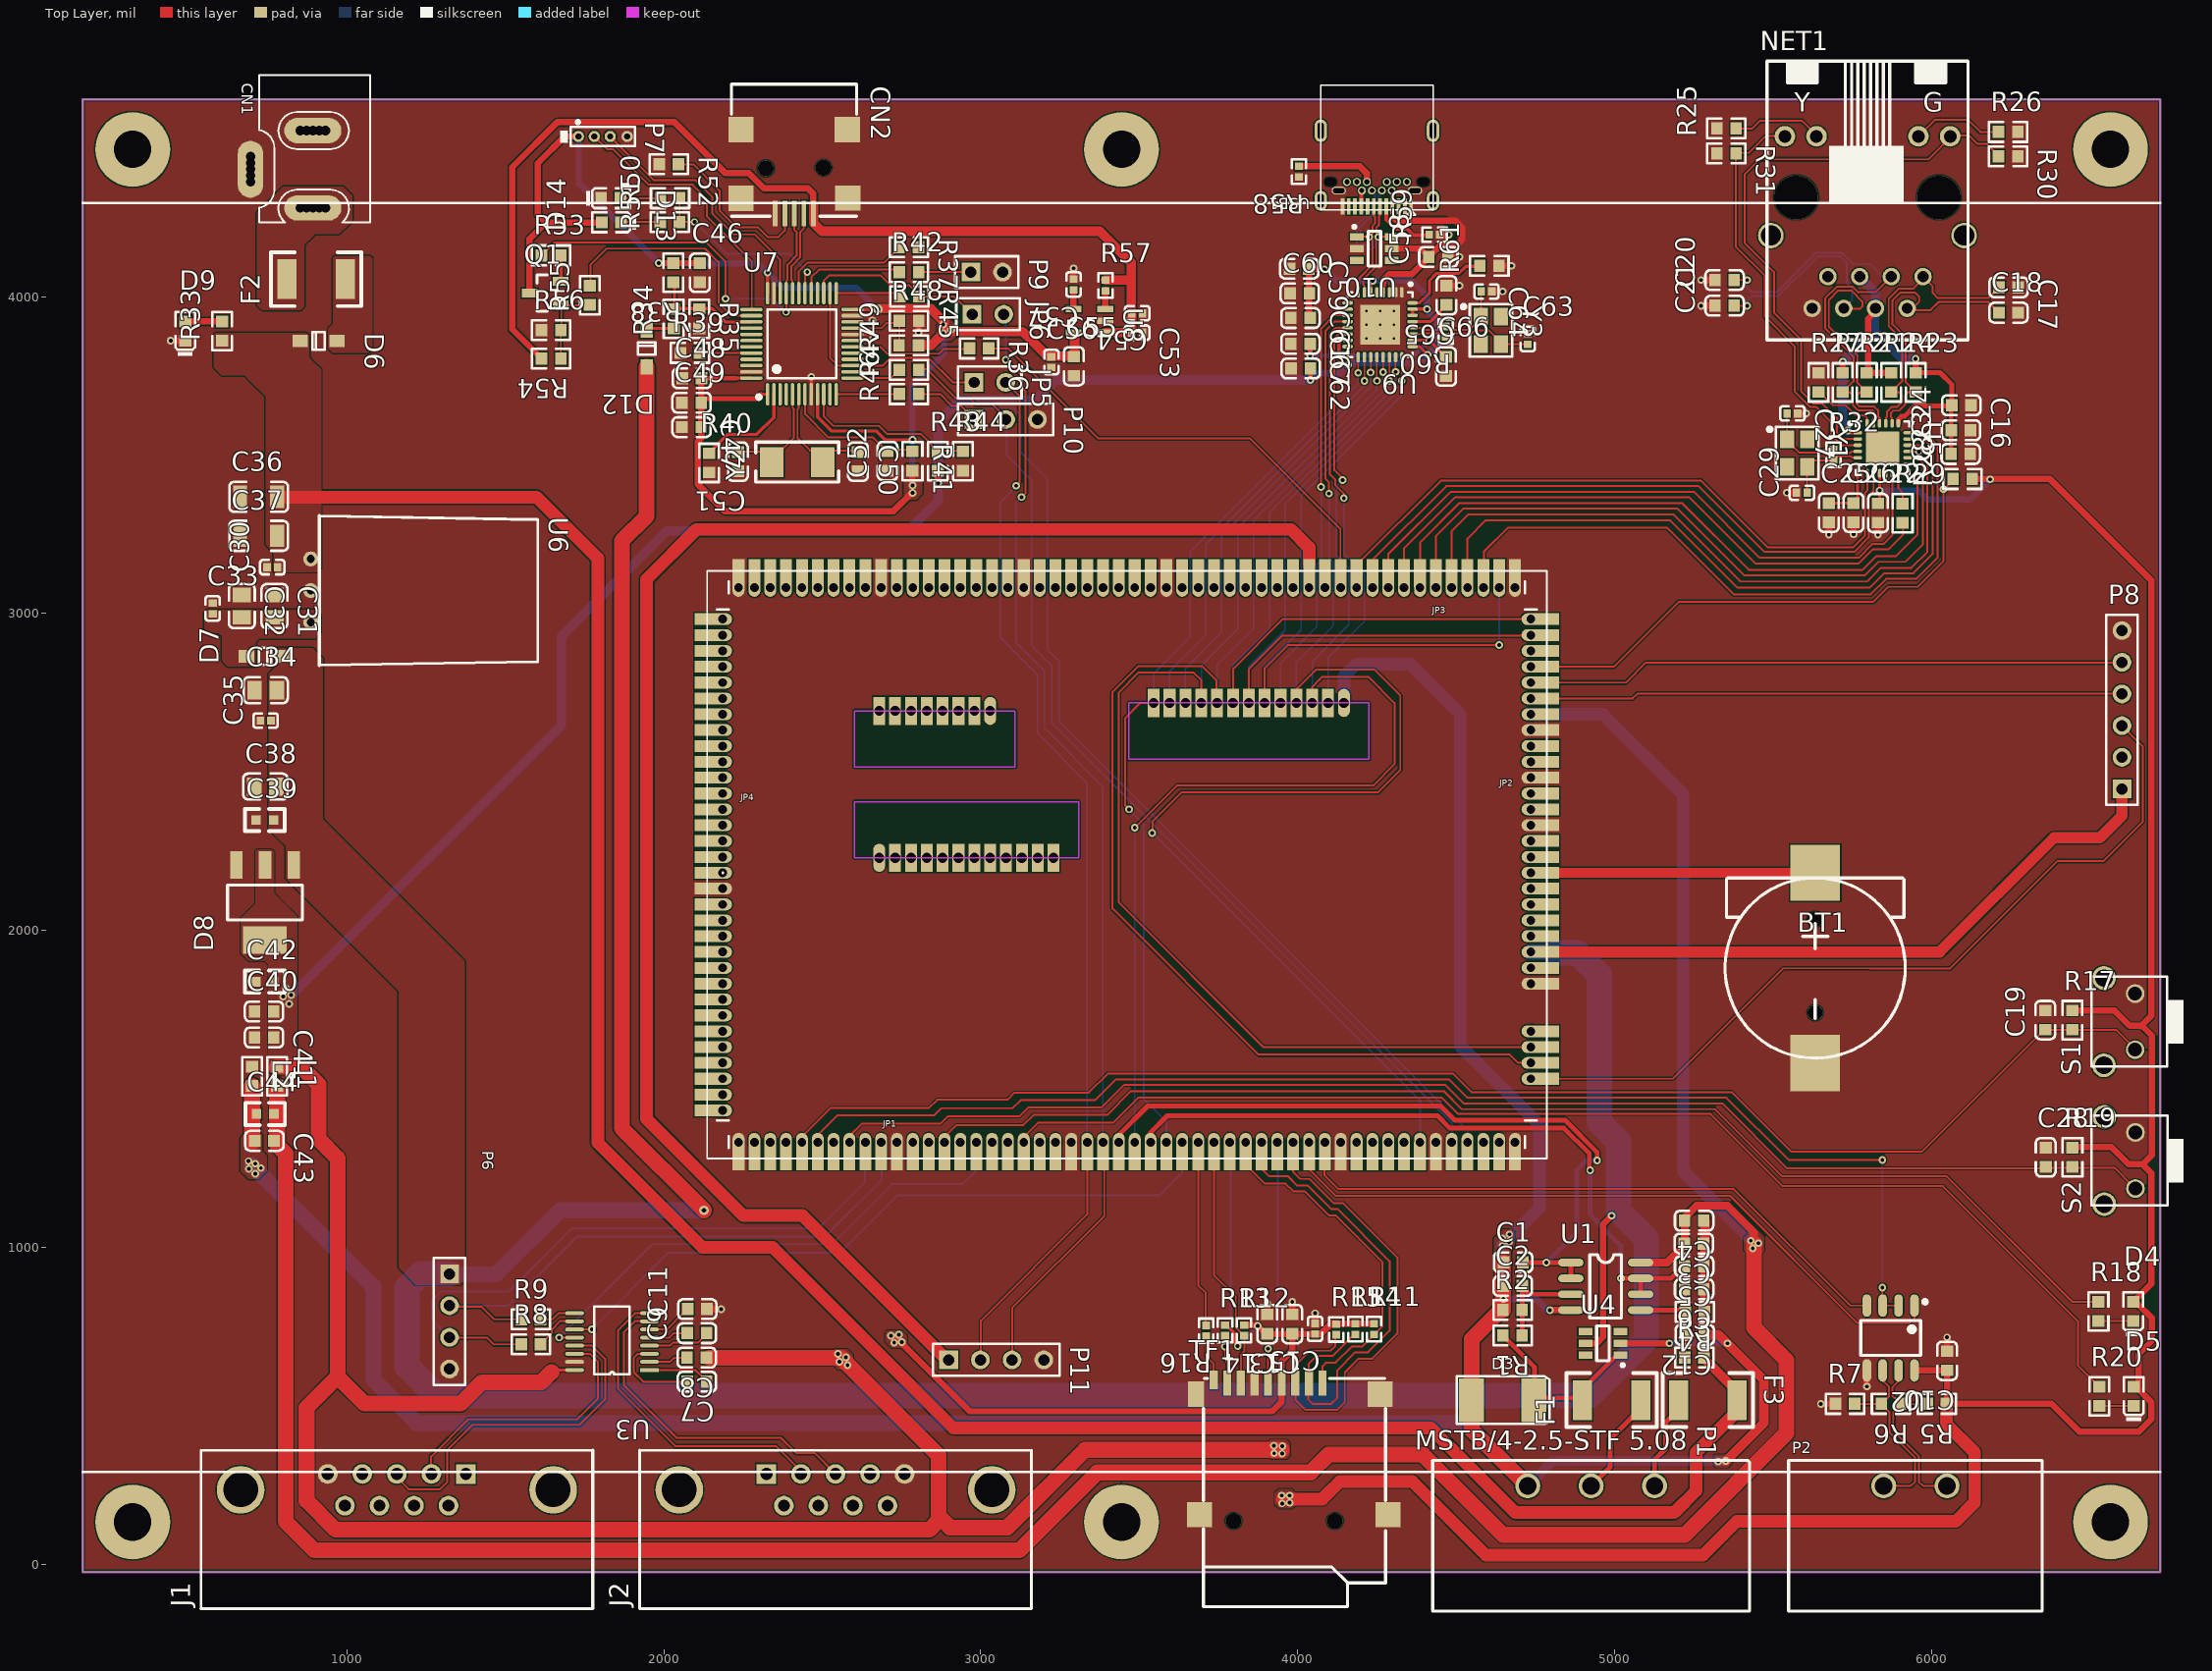
[diagram p0: Top Layer view]
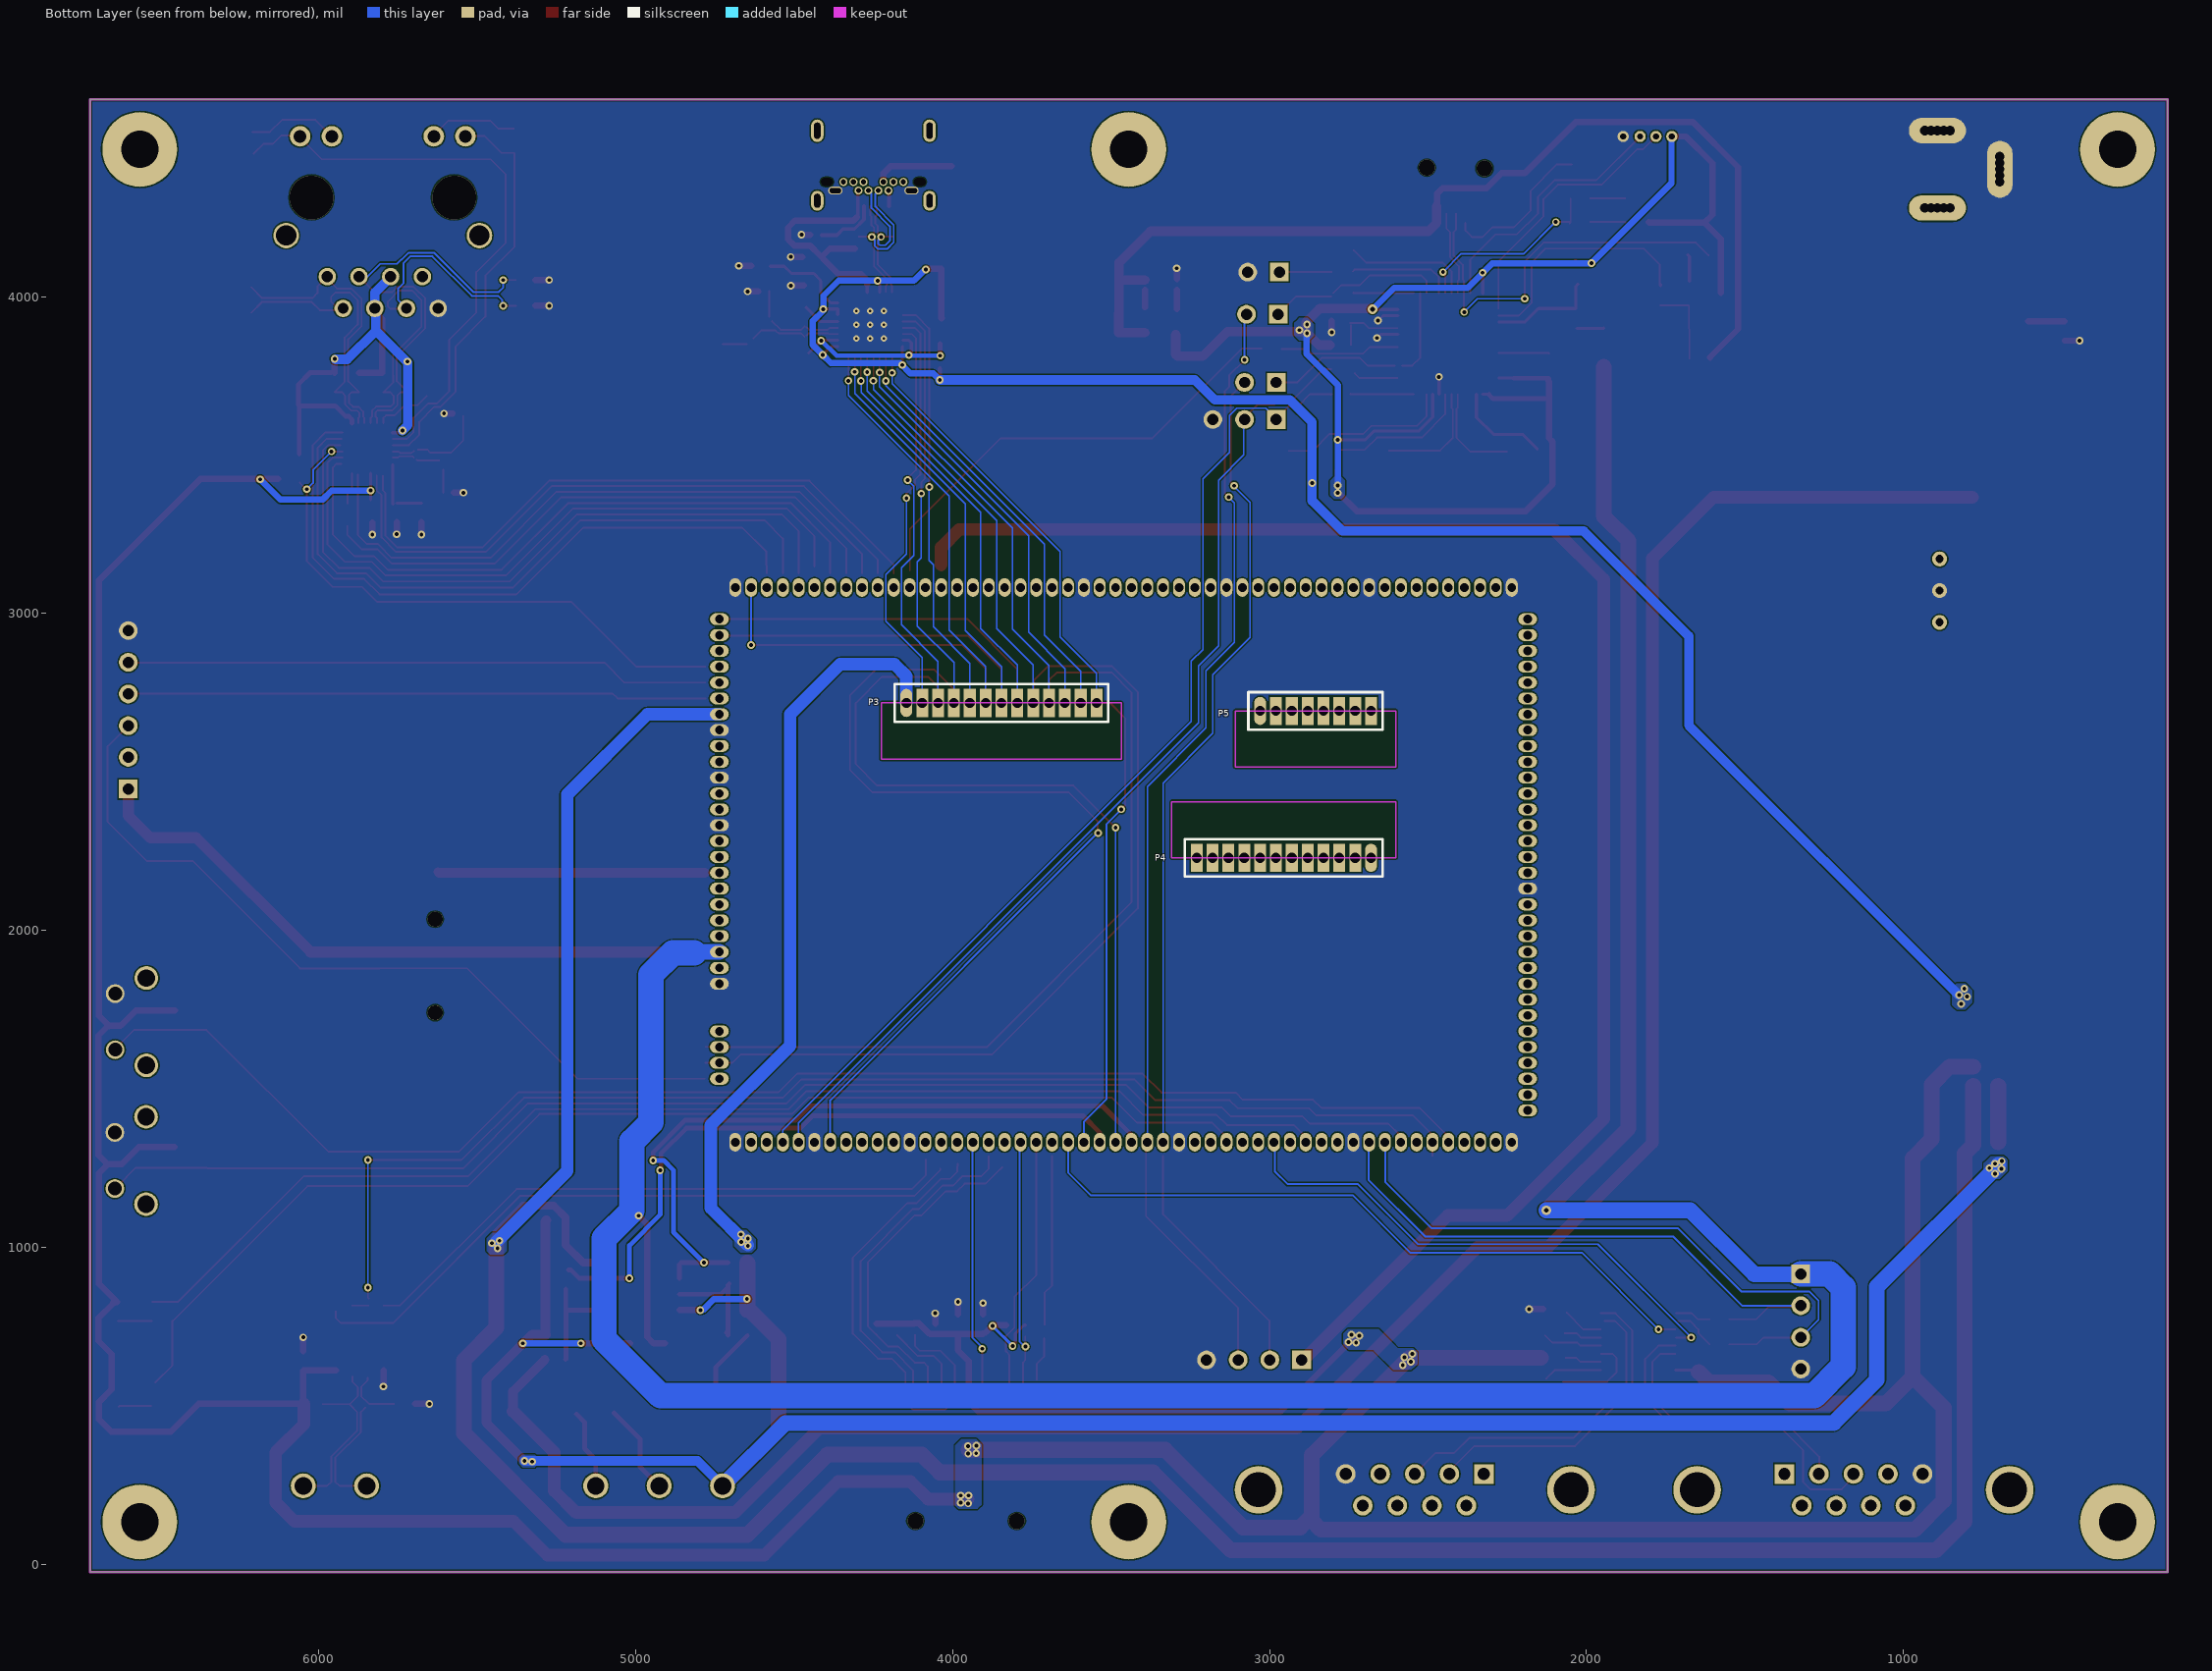
[diagram p1: Bottom Layer view, seen from below]
# Altium PCB MISC105202-15.PcbDoc (part 1 of 4)
Units mil, origin at the board's own origin, x right, y up, seen from the top; angles counter-clockwise.
Board outline 6555.12 x 4645.67 mil, 2 copper layers (Top Layer, Bottom Layer); 182 components, 258 nets, 994 pads, 145 vias.
Unrouted connection lines stored in the file: 1.

## Layer stack, top to bottom (the 12.6 mil dielectric is the usual default, probably not edited)
Top Layer: signal copper 1.4
Dielectric: dielectric 12.6, FR-4, Dk 4.8
Bottom Layer: signal copper 1.4

## Board outline
167,-24 167,4621.67 6722.12,4621.67 6722.12,-24

## Design rules (kind name [scope] priority, off if disabled: settings)
Clearance [All] p1: gap=4
ComponentClearance [All] p1: gap=10 collisioncheckmode=3 verticalgap=0 showdistances=FALSE
DiffPairsRouting [All] p1: maxlimit=6 minlimit=6 mostfreqgap=6 maxuncoupledlength=500
FanoutControl Fanout_Small [All] p1 off: bgadir=Out bgaviamode=Centered fanoutstyle=Auto fanoutdirection=Alternating viagrid=1 // Protel DXP Scope 1 Expression Was: (CompPinCount < 5)   Fanout_Small (Default Rule)
FanoutControl Fanout_Default [All] p2: bgadir=Out bgaviamode=Centered fanoutstyle=Auto fanoutdirection=Alternating viagrid=1 // Fanout_Default (Default Rule)
FanoutControl Fanout_SOIC [All] p3 off: bgadir=Out bgaviamode=Centered fanoutstyle=Auto fanoutdirection=Alternating viagrid=1 // Protel DXP Scope 1 Expression Was: IsSOIC   Fanout_SOIC (Default Rule)
FanoutControl Fanout_BGA [All] p4 off: bgadir=Out bgaviamode=Centered fanoutstyle=Auto fanoutdirection=Alternating viagrid=1 // Protel DXP Scope 1 Expression Was: IsBGA   Fanout_BGA (Default Rule)
FanoutControl Fanout_LCC [All] p5 off: bgadir=Out bgaviamode=Centered fanoutstyle=Auto fanoutdirection=Alternating viagrid=1 // Protel DXP Scope 1 Expression Was: IsLCC   Fanout_LCC (Default Rule)
MatchedLengths "Schematic Matched Net Lengths_8" [InNet('TD_N')] p1: tolerance=100 checknetsindiffpair=TRUE checkdiffpairvsdiffpair=TRUE checkothers=TRUE
MatchedLengths "Schematic Matched Net Lengths_7" [InNet('TD_N')] p2: tolerance=100 checknetsindiffpair=TRUE checkdiffpairvsdiffpair=TRUE checkothers=TRUE
MatchedLengths "Schematic Matched Net Lengths_6" [InNet('TD_N')] p3: tolerance=100 checknetsindiffpair=TRUE checkdiffpairvsdiffpair=TRUE checkothers=TRUE
MatchedLengths "Schematic Matched Net Lengths_5" [InNet('TD_P')] p4: tolerance=100 checknetsindiffpair=TRUE checkdiffpairvsdiffpair=TRUE checkothers=TRUE
MatchedLengths "Schematic Matched Net Lengths_4" [InNet('TD_P')] p5: tolerance=100 checknetsindiffpair=TRUE checkdiffpairvsdiffpair=TRUE checkothers=TRUE
MatchedLengths "Schematic Matched Net Lengths_3" [InNet('TD_N')] p6: tolerance=100 checknetsindiffpair=TRUE checkdiffpairvsdiffpair=TRUE checkothers=TRUE
MatchedLengths "Schematic Matched Net Lengths_2" [InNet('TD_N')] p7: tolerance=100 checknetsindiffpair=TRUE checkdiffpairvsdiffpair=TRUE checkothers=TRUE
MatchedLengths "Schematic Matched Net Lengths_1" [InNet('RD_P')] p8: tolerance=100 checknetsindiffpair=TRUE checkdiffpairvsdiffpair=TRUE checkothers=TRUE
MatchedLengths "Schematic Matched Net Lengths" [InNet('RD_N')] p9: tolerance=100 checknetsindiffpair=TRUE checkdiffpairvsdiffpair=TRUE checkothers=TRUE
MinimumSolderMaskSliver [All] p1: minsoldermaskwidth=0
PolygonConnect [All] p1: connectstyle=Direct reliefconductorwidth=10 reliefentries=4 polygonreliefangle="90 Angle"
RoutingVias [All] p1: holewidth=12 width=24 viastyle="Through Hole" minholewidth=12 minwidth=24 maxholewidth=12 maxwidth=24
SilkToSilkClearance [All] p1: silktosilkclearance=0
SilkscreenOverComponentPads SilkToSolderMaskClearance [IsPad] p1 off: minsilkscreentomaskgap=0 // Protel DXP Scope 1 Expression Was: IsPad
SolderMaskExpansion [All] p1: expansion=4
Width [All] p1: maxlimit=80 minlimit=4 preferedwidth=6 toplayer_minwidth=6 minimp=50.000000 maximp=50.000000 favimp=50.000000
18 further rules are at their usual default settings.

## Classes and differential pairs
component class ADC_Exp: C1 C2 C3 C4 C5 C6 C12 D3 F1 F3 P1 R1 R2 R3 R4 U1 U4
component class Connect: C7 C8 C9 C10 C11 C13 C14 C15 J1 J2 P2 P6 R5 R6 R7 R8 R9 R11 R12 R13 R14 R15 R16 TF1 U2 U3
component class Core: C19 C28 D4 D5 JP1 JP2 JP3 JP4 P3 P4 P5 P8 P11 R17 R18 R19 R20 S1 S2
component class Ethernet: C16 C17 C18 C20 C21 C22 C23 C24 C25 C26 C27 C29 NET1 R21 R22 R23 R24 R25 R26 R27 R28 R29 R30 R31 R32 U5 Y1
component class PWR: BT1 C30 C31 C32 C33 C34 C35 C36 C37 C38 C39 C40 C41 C42 C43 C44 CN1 D6 D7 D8 D9 F2 L1 L2 R33 U6
component class ST_Link: C46 C47 C48 C49 C50 C51 C52 C53 C54 C55 C56 C57 CN2 D12 D13 D14 JP5 JP6 P7 P9 P10 Q1 R34 R35 R36 R37 R38 R39 R40 R41 R42 R43 R44 R45 R46 R47 R48 R49 R50 R51 R52 R53 R54 R55 R56 R57 U7 U8 Y2
component class USB: C58 C59 C60 C61 C62 C63 C64 C65 C66 C67 R58 R59 R60 R61 U9 U10 USB1 Y3
differential pair NewDifferentialPair3: +DSI_CK_N -DSI_CK_P
differential pair NewDifferentialPair2: +D_N -D_P
differential pair NewDifferentialPair1: +RS485_A -RS485_B
differential pair RD: +RD_P -RD_N
differential pair TD: +TD_P -TD_N
differential pair NewDifferentialPair4: +STLINK_USB_DM -STLINK_USB_DP

## Components (designator, comment, footprint, x,y, rotation, side; value= is the part's Value field where it differs from the comment)
BT1 "CR2032-3V" BT1 5621,1862 r90 top
C1 "100pF,50V" 0603_C 4680,953 r0 top
C2 "100pF,50V" 0603_C 4679,878 r0 top
C3 "10uF,10V" 0603_C 5250,1012 r180 top
C4 "100nF,50V" 0603_C 5251,1084 r180 top
C5 "100pF,50V" 0603_C 5251,940 r180 top
C6 "100pF,50V" 0603_C 5251,868 r180 top
C7 "0.1uF" 0603_C 2105,576 r180 top
C8 "0.1uF" 0603_C 2104,652 r180 top
C9 "0.1uF" 0603_C 2105,729 r180 top
C10 "100nF" 0603_C 6049,642 r270 top
C11 "0.1uF" 0603_C 2106,805 r180 top
C12 "10uF,10V" 0603_C 5253,724 r180 top
C13 "22uF,6.3V" 0603_C 3983,758 r270 top
C14 "22uF,6.3V" 0603_C 3904,758 r270 top
C15 "100nF" 0402_C 4055,743 r270 top
C16 "22nF" 0603_C 6094,3657 r0 top
C17 "10pF" 0603_C 6243,4029 r0 top
C18 "10pF" 0603_C 6243,3949 r0 top
C19 "10nF" 0603_C 6359,1717 r90 top
C20 "10pF" 0603_C 5347,4052 r180 top
C21 "10pF" 0603_C 5347,3971 r180 top
C22 "100nF" 0603_C 5831,3317 r90 top
C23 "100nF" 0603_C 6092,3503 r180 top
C24 "100nF" 0603_C 6093,3578 r180 top
C25 "10uF" 0603_C 5676,3318 r90 top
C26 "100nF" 0603_C 5754,3318 r90 top
C27 "20pF" 0402_C 5561,3631 r0 top
C28 "10nF" 0603_C 6360,1284 r90 top
C29 "20pF" 0402_C 5591,3381 r180 top
C30 "0.1uF" 0402_C 765,3146 r180 top
C31 "22uF,25V" 0805_C 772,3023 r270 top
C32 "22uF,25V" 0805_C 669,3023 r270 top
C33 "0.1uF" 0402_C 577,3016 r90 top
C34 "22uF,25V" 0805_C 744,2758 r0 top
C35 "0.1uF" 0402_C 744,2662 r180 top
C36 "10uF,50V" 1206_C 722,3368 r0 top
C37 "10uF,50V" 1206_C 722,3245 r0 top
C38 "22uF,25V" 0805_C 743,2454 r0 top
C39 "0.1uF" 0603 714,2348 r0 top
C40 "22uF,6.3V" 0603_C 739,1744 r0 top
C41 "22uF,6.3V" 0603_C 739,1662 r0 top
C42 "0.1uF" 0603 714,1838 r0 top
C43 "22uF,6.3V" 0603_C 740,1336 r0 top
C44 "0.1uF" 0603 715,1421 r0 top
C46 "100nF" 0603_C 2114,4075 r90 top
C47 "100nF" 0603_C 2088,3588 r0 top
C48 "100nF" 0603_C 2089,3742 r0 top
C49 "100nF" 0603_C 2088,3665 r0 top
C50 "20pF" 0603_C 2613,3479 r270 top
C51 "20pF" 0603_C 2234,3479 r270 top
C52 "100nF" 0603_C 2706,3481 r90 top
C53 "0.1uF" 0402_C 3494,3886 r0 top
C54 "10uF" 0402_C 3494,3947 r180 top
C55 "0.1uF,25V" 0603_C 3294,3780 r90 top
C56 "10uF, 6.3V" 0402_C 3223,3793 r90 top
C57 "0.1uF" 0402_C 3293,4038 r270 top
C58 "100nF" 0603_C 4444,4125 r180 top
C59 "100nF" 0603_C 4005,4088 r0 top
C60 "100nF" 0603_C 4007,4010 r0 top
C61 "100nF" 0603_C 4009,3932 r0 top
C62 "100nF" 0603_C 4010,3773 r0 top
C63 "20pF" 0402_C 4726,3866 r90 top
C64 "20pF" 0402_C 4596,4016 r0 top
C65 "100nF" 0603_C 4470,4004 r270 top
C66 "100nF" 0603_C 4468,3779 r90 top
C67 "100nF" 0603_C 4009,3851 r0 top
CN1 "DC-10B" DC10B 893,4523.63 r270 top
CN2 "MiniUSB" Mini-USB-AB 2242,4524.63 r270 top
D3 "P6SMB6.8CA" P6KESMD 4549,518 r0 top (schematic designator D8)
D4 "green LED 0603" 0603_LED_S1 6636,797.56 r90 top
D5 "red LED 0603" 0603_LED_S1 6638,529.68 r90 top
D6 "B5819W  SL" SOD-123 911,3860 r0 top
D7 "B5819W  SL" SOD-123 742,2865 r180 top
D8 "CL1117-3.3" SOT-223 742,2088 r90 top
D9 "RED" 0603_LED_S1 490,3891 r90 top
D12 "B5819W  SL" SOD-123 1946,3836 r270 top
D13 "red LED 0603" 0603_LED_S1 1833,4310 r0 top
D14 "green LED 0603" 0603_LED_S1 1835,4234 r180 top
F1 "SMD1812P050TF/30" 1812 5083,518 r180 top
F2 "SMD1812P050TF/30" 1812 996,4055 r180 top
F3 "SMD1812P050TF/30" 1812 5202,518 r0 top
J1 "DB9F" DB9RA/F 1376,285 r180 top
J2 "DB9M" DB9RA/M 2324,285 r180 top
JP1 "Header 50" SIP-50-1.27-SMD-H-R 2236,1331.87 r90 top locked
JP2 "Header 32" SIP-32-1.27-SMD-H-R 4736,1431.87 r180 top locked
JP3 "Header 50" SIP-50-1.27-SMD-H 2236,3081.87 r90 top locked
JP4 "Header 32" SIP-32-1.27-SMD-H 2186,1431.87 r180 top locked
JP5 "" HDR1X2 2979,3729 r0 top
JP6 "" HDR1X2 2973,3944 r0 top
L1 "4.7uH ±10%" 0603_L 780,1540 r270 top
L2 "4.7uH ±10%" 0603_L 701,1540 r270 top
NET1 "HR911105A" RJ45 5798,4312.63 r0 top
P1 "SENSOR" 5.08*3B 4926,247.37 r0 top
P2 "RS485" 508*2B 5949,247.37 r0 top (schematic designator P4)
P3 "Header 13" CN13SM 4146,2717.62 r180 bottom locked
P4 "Header 12" CN12SM 2680,2229 r0 bottom locked
P5 "Header 8" CN8SM 3030,2692.62 r180 bottom locked
P6 "UART7" HDR1X4 1324,916 r270 top (schematic designator P4)
P7 "STLK_SWD" 127*4 1731,4505 r0 top
P8 "SPI2" HDR1X6 6601,2446 r90 top
P9 "MCO" HDR1X2 2969,4077 r0 top
P10 "UART1" HDR1X3 2979,3612 r0 top
P11 "TSWD" HDR1X4 2899,645 r0 top
Q1 "SS8050 Y1" SOT-23(SOT-23-3) 1626,4011 r0 top
R1 "10KΩ" 0603_R 4678,722 r180 top
R2 "10KΩ" 0603_R 4678,802 r0 top
R3 "1MΩ" 0603_R 5252,652 r0 top
R4 "100KΩ" 0603_R 5253,796 r180 top
R5 "360Ω" 0603_R 6017,506 r180 top
R6 "120Ω" 0603_R 5872,506 r180 top
R7 "360Ω" 0603_R 5727,506 r0 top
R8 "100Ω" 0603_R 1581,694 r0 top
R9 "100Ω" 0603_R 1581,773 r0 top
R11 "47K" 0402_R 4241,742 r90 top
R12 "47K" 0402_R 3831,738 r90 top
R13 "47K" 0402_R 3771,738 r90 top
R14 "47K" 0402_R 4182,742 r90 top
R15 "47K" 0402_R 4122,741 r90 top
R16 "100Ω" 0402_R 3711,737 r270 top
R17 "10K" 0603_R 6444,1717 r90 top
R18 "680Ω" 0603_R 6527,798 r90 top
R19 "10K" 0603_R 6445,1284 r90 top
R20 "680Ω" 0603_R 6529,530 r90 top
R21 "49.9Ω" 0603_R 5796,3729 r90 top
R22 "49.9Ω" 0603_R 5720,3729 r90 top
R23 "49.9Ω" 0603_R 5950,3729 r90 top
R24 "49.9Ω" 0603_R 5873,3729 r90 top
R25 "510Ω" 0603_R 5353,4530 r180 top
R26 "510Ω" 0603_R 6242,4519 r0 top
R27 "12.1KΩ" 0603_R 5644,3729 r90 top
R28 "10KΩ" 0603_R 6098,3424 r180 top
R29 "510Ω" 0603_R 5909,3316 r90 top
R30 "10KΩ" 0603_R 6242,4442 r0 top
R31 "10KΩ" 0603_R 5353,4452 r0 top
R32 "1M" 0402_R 5691,3501 r90 top
R33 "10K" 0603_R 607,3891 r90 top
R34 "2K7" 0603_R 2031,3930 r90 top
R35 "4K7" 0603_R 2112,3930 r270 top
R36 "100" 0603_R 2995,3836 r0 top
R37 "100" 0603_R 2773,4156 r0 top
R38 "10K" 0603_R 2030,4075 r270 top
R39 "100K" 0603_R 2083,3822 r0 top
R40 "10K" 0603_R 2143,3475 r90 top
R41 "100K" 0603_R 2785,3481 r270 top
R42 "100" 0603_R 2774,4077 r0 top
R43 "4K7" 0603_R 2865.43,3480.63 r90 top
R44 "4K7" 0603_R 2944,3481 r90 top
R45 "100" 0603_R 2775,4000 r0 top
R46 "100" 0603_R 2774,3692 r180 top
R47 "100" 0603_R 2774,3769 r180 top
R48 "[N/A]" 0603_R 2774,3923 r0 top
R49 "[N/A]" 0603_R 2773,3846 r180 top
R50 "510Ω" 0603_R 2020,4310 r180 top
R51 "510Ω" 0603_R 2019,4235 r180 top
R52 "100KΩ" 0603_R 2016,4417 r0 top
R53 "1K5" 0603_R 1645,4130 r0 top
R54 "10K" 0603_R 1645,3804 r180 top
R55 "100" 0603_R 1767,4004 r90 top
R56 "36K" 0603_R 1645,3894 r0 top
R57 "10K" 0402_R 3394,4035 r90 top
R58 "5K1" 0402_R 4004,4394 r270 top
R59 "5K1" 0402_R 4432,4195 r180 top
R60 "1MΩ" 0402_R 4467,3889 r270 top
R61 "12KΩ" 0603_R 4605,4097 r180 top
S1 "F1" Reset_TE 6544,1712 r90 top
S2 "F1" Reset_TE 6545,1274 r90 top
TF1 "TF" MICROSD 4057,128.37 r0 top
U1 "LM358" SO-8 4862,952 r0 top
U2 "SP3485EN-L/TR" SOIC-8_150mil 5871,714 r180 top
U3 "SP3232EEY-L/TR" TSSOP-16 1955,613 r180 top
U4 "SRV05-4-P-T7" SOT-23-6 4963,697 r0 top
U5 "LAN8720A" QFN-24_4X4x05P 5846,3521 r270 top
U6 "ZY7805LS-1000" ZY78xxLS-1000 886,3072 r270 top
U7 "STM32F103CBT6" LQFP-48_7x7x05P 2436,3851 r0 top
U8 "SP6205-3.3" SOT23-5 3293,3961 r270 top
U9 "USB330" QFN-32_5x5x05P 4260,3911 r180 top
U10 "TPD4E001DBVR" SOT-23-6 4242,4151 r180 top
USB1 "USB_TypeC_Receptacle" USB_TYPEC 4250,4412.63 r180 top
Y1 "25MHz 12PF" SMD-3225_4P 5576,3506 r270 top
Y2 "8MHz" SMD-5032_2P 2421,3478 r180 top
Y3 "24MHz" SMD-3225_4P 4610,3893 r270 top

## Footprints (in the part's own frame and the unit in brackets; to place one, negate y for a bottom-side part, rotate by r counter-clockwise, add the part's x,y. Pads: shape width x height; smd on the part's side, far side on the other; paste and mask are expansions set on the pad)
5.08*3B [mm]
  round 2 hole 1.4: 1(5.08,0) 2(0,0) 3(-5.08,0)
  silkscreen extent -12.7,-10.03 12.7,2.03
127*4 [mm]
  round 0.9 hole 0.5: 1(0,0) 2(1.27,0) 3(2.54,0) 4(3.9,0)
  silkscreen extent -1.48,-0.75 4.52,1.28
0402_C [mm]
  rect 0.6x0.65 smd mask+0.051: 1(-0.425,0) 2(0.425,0)
  silkscreen extent -0.97,-0.58 0.97,0.58, body extent -0.48,-0.3 0.52,0.3, height 0.2
0402_R [mm]
  rect 0.6x0.65 smd mask+0.051: 1(-0.425,0) 2(0.425,0)
  silkscreen extent -0.97,-0.58 0.97,0.58, body extent -0.57,-0.27 0.58,0.28, height 0.41
508*2B [mm]
  round 2 hole 1.4: 1(-2.54,0) 2(2.54,0)
  silkscreen extent -10.16,-10.03 10.16,2.03
0603 [mil]
  rect 30x30 smd: 1(0,0) 2(55,0)
  silkscreen extent -35,-35 90,35
0603_C [mm]
  rect 0.93x0.98 smd: 1(-0.77,0) 2(0.77,0)
  silkscreen extent -1.53,-0.79 1.54,0.79, body extent -0.8,-0.4 0.8,0.4, height 0.3
0603_L [mm]
  rect 0.93x0.98 smd: 1(-0.77,0) 2(0.77,0)
  silkscreen extent -1.53,-0.79 1.54,0.79, body extent -0.82,-0.41 0.82,0.41, height 0.46
0603_LED_S1 [mm]
  rect 0.93x0.98 smd: A(0.77,0) K(-0.77,0)
  silkscreen extent -1.98,-0.79 1.54,0.79, body extent -0.8,-0.4 0.8,0.4, height 0.6
0603_R [mm]
  rect 0.93x0.98 smd: 1(-0.77,0) 2(0.77,0)
  silkscreen extent -1.53,-0.79 1.54,0.79, body extent -0.85,-0.4 0.85,0.4, height 0.56
0805_C [mm]
  rect 1.16x1.47 smd: 1(-0.89,0) 2(0.89,0)
  silkscreen extent -1.77,-1.04 1.77,1.04, body extent -1,-0.63 1,0.63, height 0.77
1206_C [mm]
  rect 1.13x1.8 smd: 1(-1.49,0) 2(1.49,0)
  silkscreen extent -2.36,-1.2 2.35,1.2, body extent -1.6,-0.81 1.6,0.79, height 1
1812 [mil]
  rect 60x125 smd: 1(0,0) 2(185,0)
  silkscreen extent -50,-85 235,85
BT1 [mm]
  round 1.2 hole 1.2: 0(-3.089,-0.302) 0(4.404,-0.302)
  rect 4.5x4 smd: 1(8.112,-0.302) 2(-7.128,-0.302)
  silkscreen extent -6.73,-7.52 7.71,6.91
CN8SM [mm]
  rect 0.95x1 hole 0.8: 1(0,0) 2(1.27,0) 3(2.54,0) 4(3.81,0) 5(5.08,0) 6(6.35,0) 7(7.62,0) 8(8.89,0)
  oval 0.95x2.25 all layers, no hole: 1(0,0)
  rect 0.95x2.25 all layers, no hole: 2(1.27,0) 3(2.54,0) 4(3.81,0) 5(5.08,0) 6(6.35,0) 7(7.62,0) 8(8.89,0)
  silkscreen extent -0.94,-1.5 9.83,1.5
CN12SM [mm]
  rect 0.95x1 hole 0.8: 1(0,0) 2(1.27,0) 3(2.54,0) 4(3.81,0) 5(5.08,0) 6(6.35,0) 7(7.62,0) 8(8.89,0) 9(10.16,0) 10(11.43,0) 11(12.7,0) 12(13.97,0)
  oval 0.95x2.25 all layers, no hole: 1(0,0)
  rect 0.95x2.25 all layers, no hole: 2(1.27,0) 3(2.54,0) 4(3.81,0) 5(5.08,0) 6(6.35,0) 7(7.62,0) 8(8.89,0) 9(10.16,0) 10(11.43,0) 11(12.7,0) 12(13.97,0)
  silkscreen extent -0.94,-1.5 14.91,1.5
CN13SM [mm]
  rect 0.95x1 hole 0.8: 1(0,0) 2(1.27,0) 3(2.54,0) 4(3.81,0) 5(5.08,0) 6(6.35,0) 7(7.62,0) 8(8.89,0) 9(10.16,0) 10(11.43,0) 11(12.7,0) 12(13.97,0) 13(15.24,0)
  oval 0.95x2.25 all layers, no hole: 1(0,0)
  rect 0.95x2.25 all layers, no hole: 2(1.27,0) 3(2.54,0) 4(3.81,0) 5(5.08,0) 6(6.35,0) 7(7.62,0) 8(8.89,0) 9(10.16,0) 10(11.43,0) 11(12.7,0) 12(13.97,0) 13(15.24,0)
  silkscreen extent -0.94,-1.5 16.18,1.5
DB9RA/F [mil]
  rect 62x62 hole 38: 1(0,0)
  round 62 hole 38: 2(109,0) 3(218,0) 4(327,0) 5(436,0) 6(55,100) 7(164,100) 8(273,100) 9(382,100)
  round 150 hole 110: ""(-275,50) ""(711,50)
  silkscreen extent -400,-75 836,425
DB9RA/M [mil]
  rect 62x62 hole 38: 1(0,0)
  round 62 hole 38: 2(-109,0) 3(-218,0) 4(-327,0) 5(-436,0) 6(-55,100) 7(-164,100) 8(-273,100) 9(-382,100)
  round 150 hole 110: ""(-711,50) ""(275,50)
  silkscreen extent -836,-75 400,425
DC10B [mil]
  round 45 hole 30: 1(244.09,-40) 1(244.09,-20) 1(244.09,20) 1(244.09,40) 2(82.05,-196.85) 2(102.05,-196.85) 2(142.05,-196.85) 2(162.05,-196.85) 3(0,40) 3(0,20) 3(0,-20) 3(0,-40)
  oval 80x180 hole 30: 1(244.1,0) 3(0,0)
  oval 180x80 hole 30: 2(122.05,-196.85)
  silkscreen extent -175,-170 290,180
HDR1X2 [mm] "Connector; Header; 2 Position"
  rect 1.5x1.5 hole 0.9: 1(0,0)
  round 1.5 hole 0.9: 2(2.54,0)
  silkscreen extent -1.27,-1.27 3.81,1.27
HDR1X3 [mm] "Connector; Header; 3 Position"
  rect 1.5x1.5 hole 0.9: 1(0,0)
  round 1.5 hole 0.9: 2(2.54,0) 3(5.08,0)
  silkscreen extent -1.27,-1.27 6.35,1.27
HDR1X4 [mm] "Connector; Header; 4 Position"
  rect 1.5x1.5 hole 0.9: 1(0,0)
  round 1.5 hole 0.9: 2(2.54,0) 3(5.08,0) 4(7.62,0)
  silkscreen extent -1.27,-1.27 8.89,1.27
HDR1X6 [mm] "Connector; Header; 6 Position"
  rect 1.5x1.5 hole 0.9: 1(0,0)
  round 1.5 hole 0.9: 2(2.54,0) 3(5.08,0) 4(7.62,0) 5(10.16,0) 6(12.7,0)
  silkscreen extent -1.27,-1.27 13.97,1.27
LQFP-48_7x7x05P [mm]
  oval 0.28x1.8 smd mask+0.051: 1(-2.75,-4.05) 2(-2.25,-4.05) 3(-1.75,-4.05) 4(-1.25,-4.05) 5(-0.75,-4.05) 6(-0.25,-4.05) 7(0.25,-4.05) 8(0.75,-4.05) 9(1.25,-4.05) 10(1.75,-4.05) 11(2.25,-4.05) 12(2.75,-4.05) 25(2.75,4.05) 26(2.25,4.05) 27(1.75,4.05) 28(1.25,4.05) 29(0.75,4.05) 30(0.25,4.05) 31(-0.25,4.05) 32(-0.75,4.05) 33(-1.25,4.05) 34(-1.75,4.05) 35(-2.25,4.05) 36(-2.75,4.05)
  oval 1.8x0.28 smd mask+0.051: 13(4.05,-2.75) 14(4.05,-2.25) 15(4.05,-1.75) 16(4.05,-1.25) 17(4.05,-0.75) 18(4.05,-0.25) 19(4.05,0.25) 20(4.05,0.75) 21(4.05,1.25) 22(4.05,1.75) 23(4.05,2.25) 24(4.05,2.75) 37(-4.05,2.75) 38(-4.05,2.25) 39(-4.05,1.75) 40(-4.05,1.25) 41(-4.05,0.75) 42(-4.05,0.25) 43(-4.05,-0.25) 44(-4.05,-0.75) 45(-4.05,-1.25) 46(-4.05,-1.75) 47(-4.05,-2.25) 48(-4.05,-2.75)
  silkscreen extent -3.6,-4.42 2.75,2.75
MICROSD [mil]
  rect 51.18x80 smd: 0(-376.81,408.19)
  rect 80x80 smd: 0(-366.81,28.19) 0(203.19,408.19) 0(228.19,28.19)
  rect 25.59x80 smd: 1(21.69,443.19) 2(-21.31,443.19) 3(-64.31,443.19) 4(-107.31,443.19) 5(-150.31,443.19) 6(-193.31,443.19) 7(-236.31,443.19) 8(-279.31,443.19)
  rect 25.59x60 smd: 9(-321.81,453.19)
  silkscreen extent -354,-262 221,458
Mini-USB-AB [mil]
  rect 80x80 smd: 0(-1.89,337) 0(-1.89,2) 0(214,339) 0(215,2)
  rect 80x15 smd: 1(263.09,230) 2(263.09,200) 3(263.09,170) 4(263.09,140) 5(263.09,110)
  silkscreen extent -145,-28 271,367
P6KESMD [mm]
  rect 2x3.5 smd: 1(0,0) 2(5,0)
  silkscreen extent -1.19,-1.91 6.23,1.91
QFN-24_4X4x05P [mm]
  rect 2.68x2.68 smd mask+0.051: 0(0,0)
  oval 0.28x0.7 smd mask+0.051: 1(-1.25,-2) 2(-0.75,-2) 3(-0.25,-2) 4(0.25,-2) 5(0.75,-2) 6(1.25,-2) 13(1.25,2) 14(0.75,2) 15(0.25,2) 16(-0.25,2) 17(-0.75,2) 18(-1.25,2)
  oval 0.7x0.28 smd mask+0.051: 7(2,-1.25) 8(2,-0.75) 9(2,-0.25) 10(2,0.25) 11(2,0.75) 12(2,1.25) 19(-2,1.25) 20(-2,0.75) 21(-2,0.25) 22(-2,-0.25) 23(-2,-0.75) 24(-2,-1.25)
  silkscreen extent -2.15,-2.72 2.15,2.15
QFN-32_5x5x05P [mm] "QFN, 32-Leads, Body 5.00x5.00mm, Pitch 0.50mm, Thermal Pad 3.20x3.20mm, IPC Medium Density"
  oval 0.28x0.85 smd: 1(-1.75,-2.6) 2(-1.25,-2.6) 3(-0.75,-2.6) 4(-0.25,-2.6) 5(0.25,-2.6) 6(0.75,-2.6) 7(1.25,-2.6) 8(1.75,-2.6) 17(1.75,2.6) 18(1.25,2.6) 19(0.75,2.6) 20(0.25,2.6) 21(-0.25,2.6) 22(-0.75,2.6) 23(-1.25,2.6) 24(-1.75,2.6)
  oval 0.85x0.28 smd: 9(2.6,-1.75) 10(2.6,-1.25) 11(2.6,-0.75) 12(2.6,-0.25) 13(2.6,0.25) 14(2.6,0.75) 15(2.6,1.25) 16(2.6,1.75) 25(-2.6,1.75) 26(-2.6,1.25) 27(-2.6,0.75) 28(-2.6,0.25) 29(-2.6,-0.25) 30(-2.6,-0.75) 31(-2.6,-1.25) 32(-2.6,-1.75)
  rect 3.2x3.2 smd: 33(0,0)
  silkscreen extent -2.6,-3.37 2.6,2.6, body extent -2.45,-2.45 2.45,2.45, height 0.85
Reset_TE [mm]
  round 1.9 hole 1.4: 0(-3.5,0) 0(3.5,0)
  round 1.5 hole 1.1: 1(-2.25,-2.5) 2(2.25,-2.5)
  silkscreen extent -3.6,-6.36 3.61,1.01
RJ45 [mm]
  round 2.05 hole 1.63: 0(-7.745,-3.05) 0(7.745,-3.05)
  round 1.397 hole 0.89: 1(4.45,-6.35) 2(3.18,-8.89) 3(1.91,-6.35) 4(0.64,-8.89) 5(-0.63,-6.35) 6(-1.9,-8.89) 7(-3.17,-6.35) 8(-4.44,-8.89)
  round 1.651 hole 1.016: 9(6.625,4.9) 10(4.085,4.9) 11(-4.085,4.9) 12(-6.625,4.9)
  silkscreen extent -8.05,-11.45 8.05,10.92
SIP-32-1.27-SMD-H [mm]
  oval 1.5x0.95 hole 0.7: 1(0,0) 2(0,-1.27) 3(0,-2.54) 4(0,-3.81) 5(0,-5.08) 6(0,-6.35) 7(0,-7.62) 8(0,-8.89) 9(0,-10.16) 10(0,-11.43) 11(0,-12.7) 12(0,-13.97) 13(0,-15.24) 14(0,-16.51) 15(0,-17.78) 16(0,-19.05) 17(0,-20.32) 18(0,-21.59) 19(0,-22.86) 20(0,-24.13) 21(0,-25.4) 22(0,-26.67) 23(0,-27.94) 24(0,-29.21) 25(0,-30.48) 26(0,-31.75) 27(0,-33.02) 28(0,-34.29) 29(0,-35.56) 30(0,-36.83) 31(0,-38.1) 32(0,-39.37)
  rect 2.25x0.95 smd: 1(1.13,0) 2(1.13,-1.27) 3(1.13,-2.54) 4(1.13,-3.81) 5(1.13,-5.08) 6(1.13,-6.35) 7(1.13,-7.62) 8(1.13,-8.89) 9(1.13,-10.16) 10(1.13,-11.43) 11(1.13,-12.7) 12(1.13,-13.97) 13(1.13,-15.24) 14(1.13,-16.51) 15(1.13,-17.78) 16(1.13,-19.05) 17(1.13,-20.32) 18(1.13,-21.59) 19(1.13,-22.86) 20(1.13,-24.13) 21(1.13,-25.4) 22(1.13,-26.67) 23(1.13,-27.94) 24(1.13,-29.21) 25(1.13,-30.48) 26(1.13,-31.75) 27(1.13,-33.02) 28(1.13,-34.29) 29(1.13,-35.56) 30(1.13,-36.83) 31(1.13,-38.1) 32(1.13,-39.37)
  silkscreen extent -0.47,-40.17 0.47,0.8
SIP-32-1.27-SMD-H-R [mm]
  rect 2.25x0.95 smd: 3(-1.13,-2.54) 4(-1.13,-3.81) 5(-1.13,-5.08) 6(-1.13,-6.35) 9(-1.13,-10.16) 10(-1.13,-11.43) 11(-1.13,-12.7) 12(-1.13,-13.97) 13(-1.13,-15.24) 14(-1.13,-16.51) 15(-1.13,-17.78) 16(-1.13,-19.05) 17(-1.13,-20.32) 18(-1.13,-21.59) 19(-1.13,-22.86) 20(-1.13,-24.13) 21(-1.13,-25.4) 22(-1.13,-26.67) 23(-1.13,-27.94) 24(-1.13,-29.21) 25(-1.13,-30.48) 26(-1.13,-31.75) 27(-1.13,-33.02) 28(-1.13,-34.29) 29(-1.13,-35.56) 30(-1.13,-36.83) 31(-1.13,-38.1) 32(-1.13,-39.37)
  oval 1.5x0.95 hole 0.7: 3(0,-2.54) 4(0,-3.81) 5(0,-5.08) 6(0,-6.35) 9(0,-10.16) 10(0,-11.43) 11(0,-12.7) 12(0,-13.97) 13(0,-15.24) 14(0,-16.51) 15(0,-17.78) 16(0,-19.05) 17(0,-20.32) 18(0,-21.59) 19(0,-22.86) 20(0,-24.13) 21(0,-25.4) 22(0,-26.67) 23(0,-27.94) 24(0,-29.21) 25(0,-30.48) 26(0,-31.75) 27(0,-33.02) 28(0,-34.29) 29(0,-35.56) 30(0,-36.83) 31(0,-38.1) 32(0,-39.37)
  silkscreen extent -0.47,-40.17 0.47,0.8
SIP-50-1.27-SMD-H [mm]
  oval 1.5x0.95 hole 0.7: 1(0,0) 2(0,-1.27) 3(0,-2.54) 4(0,-3.81) 5(0,-5.08) 6(0,-6.35) 7(0,-7.62) 8(0,-8.89) 9(0,-10.16) 10(0,-11.43) 11(0,-12.7) 12(0,-13.97) 13(0,-15.24) 14(0,-16.51) 15(0,-17.78) 16(0,-19.05) 17(0,-20.32) 18(0,-21.59) 19(0,-22.86) 20(0,-24.13) 21(0,-25.4) 22(0,-26.67) 23(0,-27.94) 24(0,-29.21) 25(0,-30.48) 26(0,-31.75) 27(0,-33.02) 28(0,-34.29) 29(0,-35.56) 30(0,-36.83) 31(0,-38.1) 32(0,-39.37) 33(0,-40.64) 34(0,-41.91) 35(0,-43.18) 36(0,-44.45) 37(0,-45.72) 38(0,-46.99) 39(0,-48.26) 40(0,-49.53) 41(0,-50.8) 42(0,-52.07) 43(0,-53.34) 44(0,-54.61) 45(0,-55.88) 46(0,-57.15) 47(0,-58.42) 48(0,-59.69) 49(0,-60.96) 50(0,-62.23)
  rect 2.25x0.95 smd: 1(1.13,0) 2(1.13,-1.27) 3(1.13,-2.54) 4(1.13,-3.81) 5(1.13,-5.08) 6(1.13,-6.35) 7(1.13,-7.62) 8(1.13,-8.89) 9(1.13,-10.16) 10(1.13,-11.43) 11(1.13,-12.7) 12(1.13,-13.97) 13(1.13,-15.24) 14(1.13,-16.51) 15(1.13,-17.78) 16(1.13,-19.05) 17(1.13,-20.32) 18(1.13,-21.59) 19(1.13,-22.86) 20(1.13,-24.13) 21(1.13,-25.4) 22(1.13,-26.67) 23(1.13,-27.94) 24(1.13,-29.21) 25(1.13,-30.48) 26(1.13,-31.75) 27(1.13,-33.02) 28(1.13,-34.29) 29(1.13,-35.56) 30(1.13,-36.83) 31(1.13,-38.1) 32(1.13,-39.37) 33(1.13,-40.64) 34(1.13,-41.91) 35(1.13,-43.18) 36(1.13,-44.45) 37(1.13,-45.72) 38(1.13,-46.99) 39(1.13,-48.26) 40(1.13,-49.53) 41(1.13,-50.8) 42(1.13,-52.07) 43(1.13,-53.34) 44(1.13,-54.61) 45(1.13,-55.88) 46(1.13,-57.15) 47(1.13,-58.42) 48(1.13,-59.69) 49(1.13,-60.96) 50(1.13,-62.23)
  silkscreen extent -0.47,-63.03 0.47,0.8
SIP-50-1.27-SMD-H-R [mm]
  rect 2.25x0.95 smd: 1(-1.13,0) 2(-1.13,-1.27) 3(-1.13,-2.54) 4(-1.13,-3.81) 5(-1.13,-5.08) 6(-1.13,-6.35) 7(-1.13,-7.62) 8(-1.13,-8.89) 9(-1.13,-10.16) 10(-1.13,-11.43) 11(-1.13,-12.7) 12(-1.13,-13.97) 13(-1.13,-15.24) 14(-1.13,-16.51) 15(-1.13,-17.78) 16(-1.13,-19.05) 17(-1.13,-20.32) 18(-1.13,-21.59) 19(-1.13,-22.86) 20(-1.13,-24.13) 21(-1.13,-25.4) 22(-1.13,-26.67) 23(-1.13,-27.94) 24(-1.13,-29.21) 25(-1.13,-30.48) 26(-1.13,-31.75) 27(-1.13,-33.02) 28(-1.13,-34.29) 29(-1.13,-35.56) 30(-1.13,-36.83) 31(-1.13,-38.1) 32(-1.13,-39.37) 33(-1.13,-40.64) 34(-1.13,-41.91) 35(-1.13,-43.18) 36(-1.13,-44.45) 37(-1.13,-45.72) 38(-1.13,-46.99) 39(-1.13,-48.26) 40(-1.13,-49.53) 41(-1.13,-50.8) 42(-1.13,-52.07) 43(-1.13,-53.34) 44(-1.13,-54.61) 45(-1.13,-55.88) 46(-1.13,-57.15) 47(-1.13,-58.42) 48(-1.13,-59.69) 49(-1.13,-60.96) 50(-1.13,-62.23)
  oval 1.5x0.95 hole 0.7: 1(0,0) 2(0,-1.27) 3(0,-2.54) 4(0,-3.81) 5(0,-5.08) 6(0,-6.35) 7(0,-7.62) 8(0,-8.89) 9(0,-10.16) 10(0,-11.43) 11(0,-12.7) 12(0,-13.97) 13(0,-15.24) 14(0,-16.51) 15(0,-17.78) 16(0,-19.05) 17(0,-20.32) 18(0,-21.59) 19(0,-22.86) 20(0,-24.13) 21(0,-25.4) 22(0,-26.67) 23(0,-27.94) 24(0,-29.21) 25(0,-30.48) 26(0,-31.75) 27(0,-33.02) 28(0,-34.29) 29(0,-35.56) 30(0,-36.83) 31(0,-38.1) 32(0,-39.37) 33(0,-40.64) 34(0,-41.91) 35(0,-43.18) 36(0,-44.45) 37(0,-45.72) 38(0,-46.99) 39(0,-48.26) 40(0,-49.53) 41(0,-50.8) 42(0,-52.07) 43(0,-53.34) 44(0,-54.61) 45(0,-55.88) 46(0,-57.15) 47(0,-58.42) 48(0,-59.69) 49(0,-60.96) 50(0,-62.23)
  silkscreen extent -0.47,-63.03 0.47,0.8